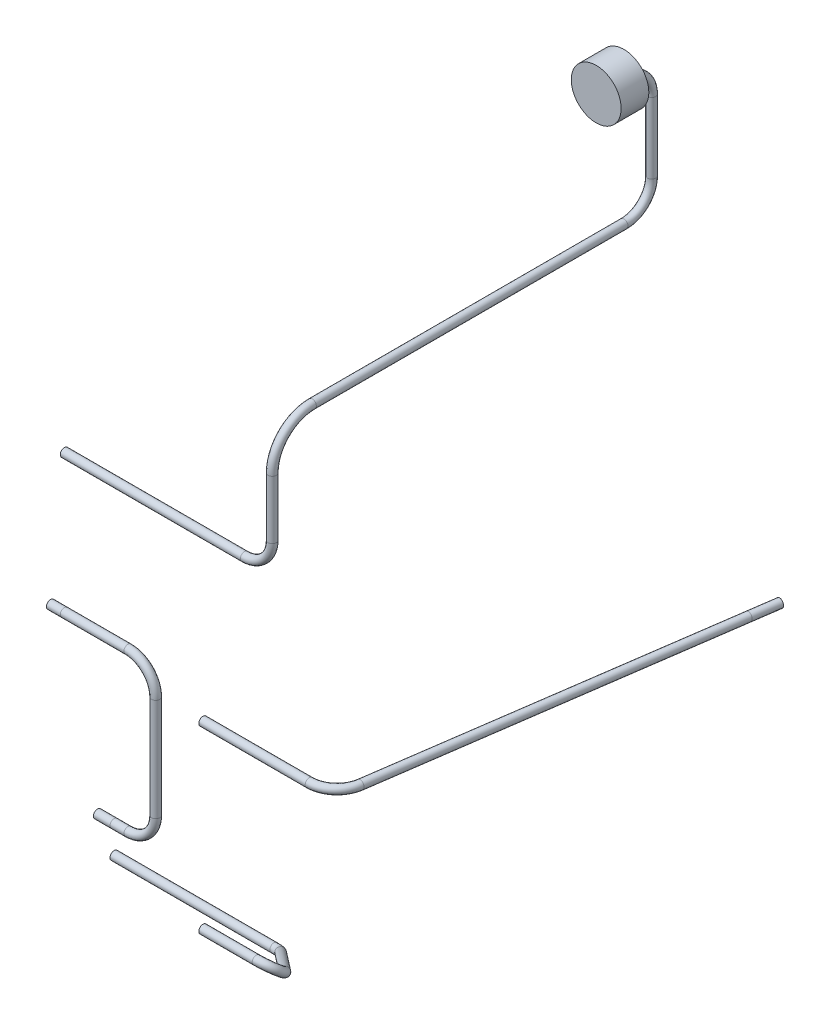
from build123d import *

# Parameters (mm, degrees)
SWEEP1_PROFILE_R    = 1.5
SWEEP2_PROFILE_R    = 1.5
SWEEP3_PROFILE_R    = 1.5
SWEEP4_PROFILE_R    = 1.5
SKETCH55_R          = 9
BOSS_EXTRUDE1_DEPTH = 10


with BuildPart() as part:
    # Sweep1: sweep along a curve in space
    with BuildLine() as sweep1_path:
        Line((-433, -499, -265), (-413.717668682, -499, -265))
        ThreePointArc((-413.717668682, -499, -265), (-409.186497243, -500.776823058, -267.274333514), (-409.88632901, -504.056041857, -271.471733577))
        Line((-409.88632901, -504.056041857, -271.471733577), (-435.551257158, -522.899601437, -295.59148984))
        ThreePointArc((-435.551257158, -522.899601437, -295.59148984), (-437.268717603, -523.71136849, -296.630551667), (-439.382596831, -524, -297))
        Line((-497.05, -524, -297), (-439.382596831, -524, -297))
    # Sweep1 profile (on start of the path) → Sweep1 (sweep)
    with BuildSketch(Plane(origin=(-433, -499, -265), x_dir=(0, 0, 1), z_dir=(1, 0, 0))):
        Circle(SWEEP1_PROFILE_R)
    sweep(path=sweep1_path.line)


with BuildPart() as body_2:
    # Sweep2: sweep along a path in Sketch2
    with BuildLine(Plane(origin=(0, 0, -297), x_dir=(-1, 0, 0), z_dir=(0, 0, -1))) as sweep2_path:
        Line((520, -457), (515, -457))
        Line((515, -457), (492.05, -457))
        ThreePointArc((492.05, -457), (484.978932188, -459.928932188), (482.05, -467))
        Line((482.05, -467), (482.05, -504))
        ThreePointArc((482.05, -504), (484.978932188, -511.071067812), (492.05, -514))
        Line((492.05, -514), (497.05, -514))
        Line((497.05, -514), (503.05, -514))
    # Sweep2 profile (on start of the path) → Sweep2 (sweep)
    with BuildSketch(Plane(origin=(-520, -457, -297), x_dir=(0, 0, 1), z_dir=(1, 0, 0))):
        Circle(SWEEP2_PROFILE_R)
    sweep(path=sweep2_path.line)


with BuildPart() as body_3:
    # Sweep3: sweep along a path in Sketch1
    with BuildLine(Plane(origin=(0, -434, 0), x_dir=(-1, 0, 0), z_dir=(0, -1, 0))) as sweep3_path:
        Line((365.770013082, 406.090418299), (367.184226644, 396.190923362))
        Line((367.184226644, 396.190923362), (384.699246205, 273.585786438))
        ThreePointArc((384.699246205, 273.585786438), (388.046723728, 267.44546045), (394.598741142, 265))
        Line((394.598741142, 265), (433, 265))
    # Sweep3 profile (on start of the path) → Sweep3 (sweep)
    with BuildSketch(Plane(origin=(-365.770013082, -434, -406.090418299), x_dir=(0.9899494936611664, 0, 0.14142135623731125), z_dir=(-0.14142135623731125, 0, 0.9899494936611664))):
        Circle(SWEEP3_PROFILE_R)
    sweep(path=sweep3_path.line)


with BuildPart() as body_4:
    # Sweep4: sweep along a curve in space
    with BuildLine() as sweep4_path:
        Line((-515, -407, -297), (-450, -407, -297))
        ThreePointArc((-450, -407, -297), (-442.928932188, -404.071067812, -297), (-440, -397, -297))
        Line((-440, -375.938087088, -297), (-440, -397, -297))
        ThreePointArc((-440, -375.938087088, -297), (-440, -365.728817801, -301.228817801), (-440, -361.5, -311.438087088))
        Line((-440, -361.5, -423.95), (-440, -361.5, -311.438087088))
        ThreePointArc((-440, -351.5, -433.95), (-440, -358.571067812, -431.021067812), (-440, -361.5, -423.95))
        Line((-440, -326, -433.95), (-440, -351.5, -433.95))
        ThreePointArc((-440, -326, -433.95), (-440, -318.928932188, -431.021067812), (-440, -316, -423.95))
        Line((-440, -316, -413.95), (-440, -316, -423.95))
    # Sweep4 profile (on start of the path) → Sweep4 (sweep)
    with BuildSketch(Plane(origin=(-515, -407, -297), x_dir=(0, 0, 1), z_dir=(1, 0, 0))):
        Circle(SWEEP4_PROFILE_R)
    sweep(path=sweep4_path.line)

    # Sketch55 → Boss-Extrude1 (add)
    with BuildSketch(Plane.XY.offset(-413.95)):
        with Locations((-440, -316)):
            Circle(SKETCH55_R)
    extrude(amount=-BOSS_EXTRUDE1_DEPTH)


solid = Compound([part.part, body_2.part, body_3.part, body_4.part])
